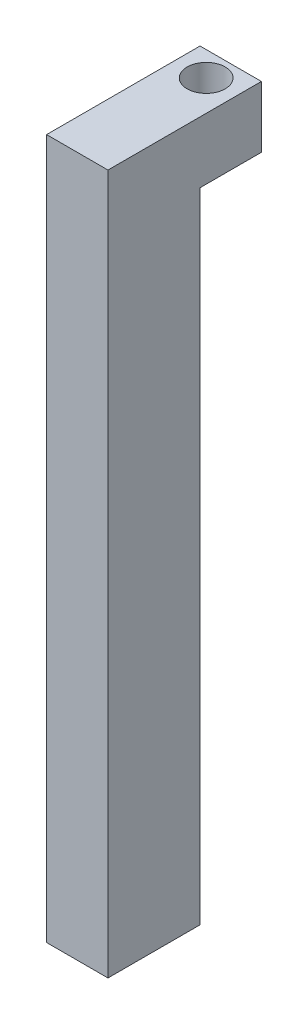
from build123d import *

# Parameters (mm, degrees)
SKETCH1_W                   = 10
SKETCH1_H                   = 15
BOSS_EXTRUDE1_DEPTH         = 114
SKETCH2_W                   = 10
SKETCH2_H                   = 10
SKETCH2_R                   = 3.1
BOSS_EXTRUDE2_DEPTH         = 10
M4_TAPPED_HOLE1_D           = 3.3
M4_TAPPED_HOLE1_DEPTH       = 11.5
M4_TAPPED_HOLE1_CSINK_D     = 4.05
M4_TAPPED_HOLE1_CSINK_ANGLE = 90
M4_TAPPED_HOLE1_TIP         = 0.991420021


with BuildPart() as part:
    # Sketch1 → Boss-Extrude1 (new body)
    with BuildSketch(Plane(origin=(0, 0, 0), x_dir=(1, 0, 0), z_dir=(0, 1, 0))):
        Rectangle(SKETCH1_W, SKETCH1_H)
    extrude(amount=BOSS_EXTRUDE1_DEPTH)

    # Sketch2 → Boss-Extrude2 (add)
    with BuildSketch(Plane(origin=(0, 114, 0), x_dir=(1, 0, 0), z_dir=(0, 1, 0))):
        with Locations((0, 12.5)):
            Rectangle(SKETCH2_W, SKETCH2_H)
        with Locations(Location((0, 13.5, 0), (0, 0, 270))):
            Circle(SKETCH2_R, mode=Mode.SUBTRACT)
    extrude(amount=-BOSS_EXTRUDE2_DEPTH)

    # M4 Tapped Hole1
    with Locations(Plane(origin=(0, 0, 0), x_dir=(-1, 0, 0), z_dir=(0, -1, 0))):
        with Locations((0, 3.5), (0, -3.5)):
            CounterSinkHole(M4_TAPPED_HOLE1_D / 2, M4_TAPPED_HOLE1_CSINK_D / 2, depth=M4_TAPPED_HOLE1_DEPTH, counter_sink_angle=M4_TAPPED_HOLE1_CSINK_ANGLE)
            with Locations((0, 0, -(M4_TAPPED_HOLE1_DEPTH + M4_TAPPED_HOLE1_TIP / 2))):  # 118° drill point
                Cone(0, M4_TAPPED_HOLE1_D / 2, M4_TAPPED_HOLE1_TIP, mode=Mode.SUBTRACT)


solid = part.part
